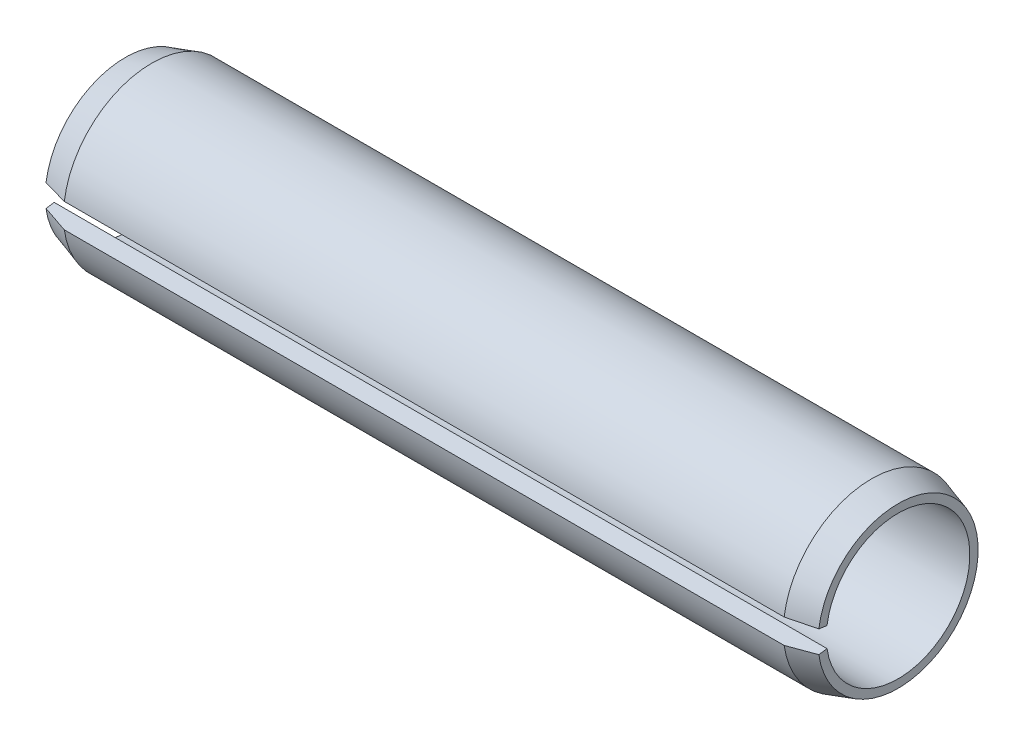
from build123d import *

# Parameters (mm, degrees)
SKETCH1_R          = 8
SKETCH1_R_2        = 7.25
BASE_EXTRUDE_DEPTH = 70
SKETCH2_R          = 7.25
SKETCH2_R_2        = 6.5
EXTRUDE2_DEPTH     = 70
GAP_DEPTH          = 71.908391605


with BuildPart() as part:
    # Sketch1 → Base-Extrude (new body)
    with BuildSketch(Plane(origin=(0, 0, 0), x_dir=(0, 0, -1), z_dir=(1, 0, 0))):
        Circle(SKETCH1_R)
        Circle(SKETCH1_R_2, mode=Mode.SUBTRACT)
    extrude(amount=BASE_EXTRUDE_DEPTH)

    # Sketch2 → Extrude2 (add)
    with BuildSketch(Plane(origin=(0, 0, 0), x_dir=(0, 0, -1), z_dir=(1, 0, 0))):
        Circle(SKETCH2_R)
        Circle(SKETCH2_R_2, mode=Mode.SUBTRACT)
    extrude(amount=EXTRUDE2_DEPTH)

    # Sketch3 → Cut-Revolve1 (revolve, cut)
    with BuildSketch(Plane.XY, mode=Mode.PRIVATE) as cut_revolve1_sk:
        Polygon((70, 8), (70, 7.25), (67.6, 8), align=None)
        Polygon((2.4, 8), (0, 7.25), (0, 8), align=None)
    revolve(cut_revolve1_sk.sketch.rotate(Axis((35, 0, 0), (-1, 0, 0)), 90), axis=Axis((35, 0, 0), (-1, 0, 0)), mode=Mode.SUBTRACT)

    # Sketch4 → Gap (cut, through all)
    with BuildSketch(Plane(origin=(0, 0, 0), x_dir=(0, 0, -1), z_dir=(1, 0, 0))):
        Polygon((0, 0), (-8.1, 1.138380761), (-8.1, -1.138380761), align=None)
    extrude(amount=GAP_DEPTH, mode=Mode.SUBTRACT)


solid = part.part
